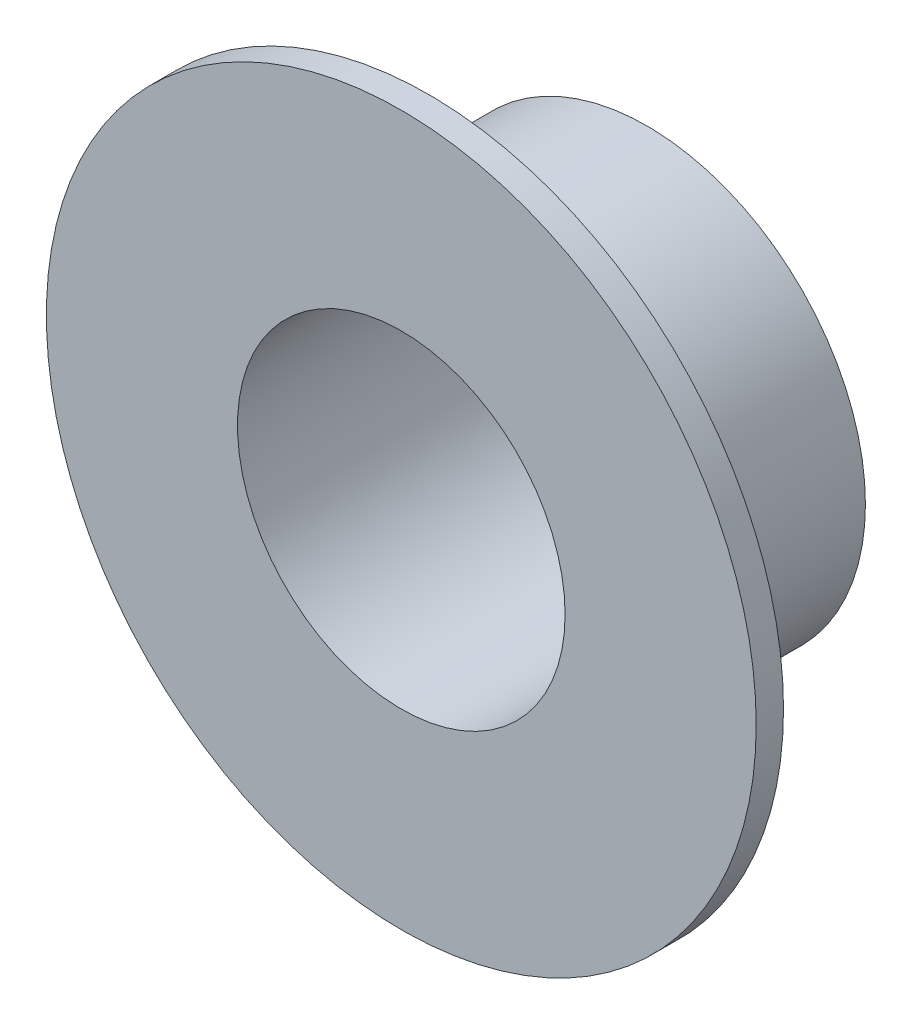
from build123d import *

# Parameters (mm, degrees)
SKETCH1_R           = 40
SKETCH1_R_2         = 30
BOSS_EXTRUDE1_DEPTH = 40
SKETCH2_R           = 65
SKETCH2_R_2         = 30
BOSS_EXTRUDE2_DEPTH = 5


with BuildPart() as part:
    # Sketch1 → Boss-Extrude1 (new body)
    with BuildSketch(Plane.XY):
        Circle(SKETCH1_R)
        Circle(SKETCH1_R_2, mode=Mode.SUBTRACT)
    extrude(amount=BOSS_EXTRUDE1_DEPTH)

    # Sketch2 → Boss-Extrude2 (add)
    with BuildSketch(Plane.XY.offset(40)):
        Circle(SKETCH2_R)
        Circle(SKETCH2_R_2, mode=Mode.SUBTRACT)
    extrude(amount=BOSS_EXTRUDE2_DEPTH)


solid = part.part
